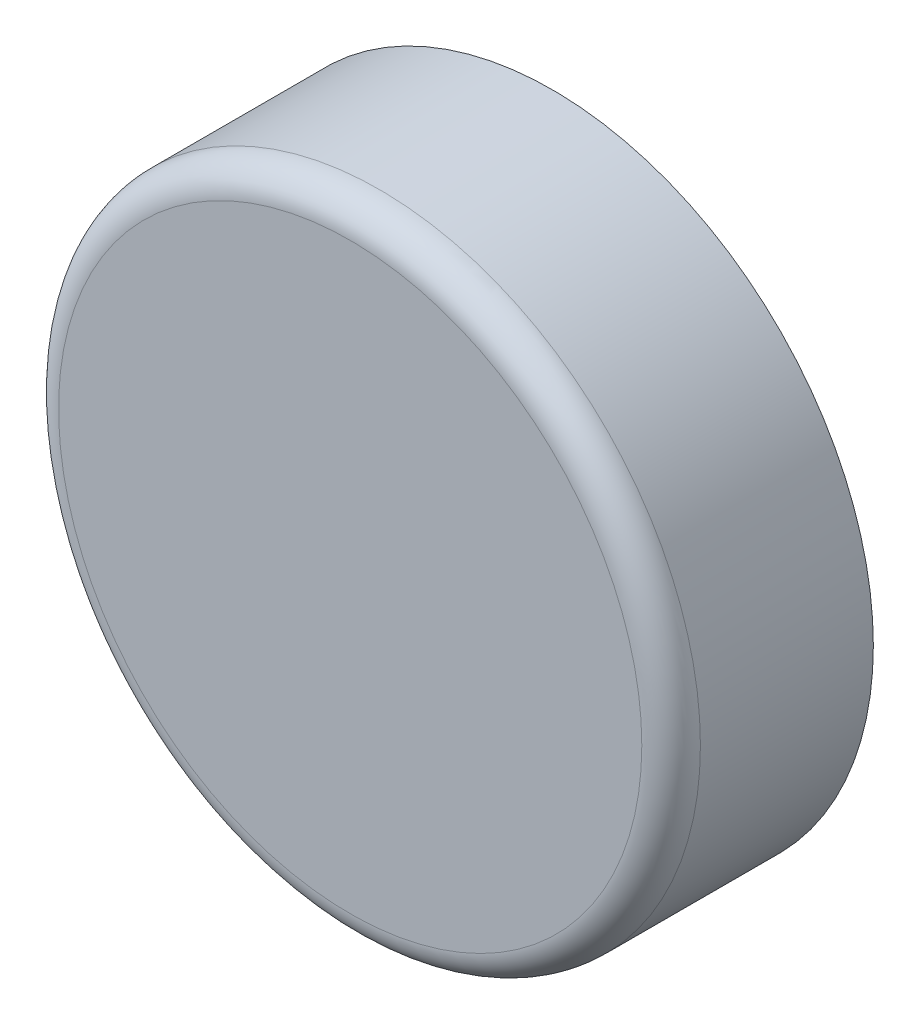
from build123d import *

# Parameters (mm, degrees)
SKETCH1_R           = 109.5
BOSS_EXTRUDE1_DEPTH = 69
SHELL1_T            = -6
FILLET1_R           = 10
FILLET2_R           = 4


with BuildPart() as part:
    # Sketch1 → Boss-Extrude1 (new body)
    with BuildSketch(Plane.XY):
        Circle(SKETCH1_R)
    extrude(amount=BOSS_EXTRUDE1_DEPTH)

    # Shell1
    shell1_openings = [part.faces().sort_by_distance(p)[0] for p in [
        (0, 0, 0),
    ]]
    offset(amount=SHELL1_T, openings=shell1_openings, kind=Kind.INTERSECTION)

    # Fillet1
    fillet1_edges = [part.edges().sort_by_distance(p)[0] for p in [
        (-109.5, 0, 69),
    ]]
    fillet(fillet1_edges, radius=FILLET1_R)

    # Fillet2
    fillet2_edges = [part.edges().sort_by_distance(p)[0] for p in [
        (-103.5, 0, 63),
    ]]
    fillet(fillet2_edges, radius=FILLET2_R)


solid = part.part
